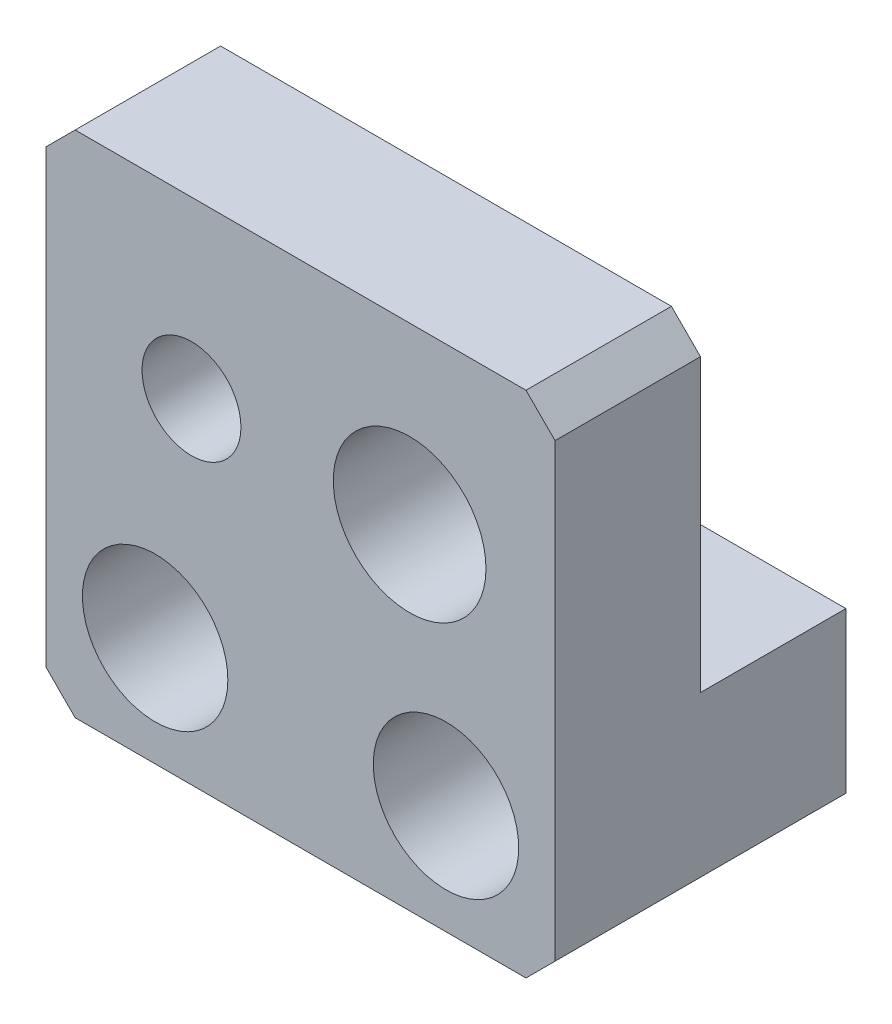
from build123d import *

# Parameters (mm, degrees)
SKETCH_1_W                   = 35
SKETCH_1_H                   = 35
EXTRUDE_1_DEPTH              = 20
CHAMFER_1_SIZE               = 2
M12X1_25_1_D                 = 10.5
HOLE_WIZARD_M8_1_D           = 6.8
HOLE_WIZARD_M5_1_D           = 5.5
HOLE_WIZARD_M5_1_CBORE_D     = 10
HOLE_WIZARD_M5_1_CBORE_DEPTH = 12
SKETCH_11_W                  = 10
SKETCH_11_H                  = 22
CUT_EXTRUDE_1_DEPTH          = 44.945989578


with BuildPart() as part:
    # 草图1 → 凸台-拉伸1 (new body)
    with BuildSketch(Plane.XY):
        Rectangle(SKETCH_1_W, SKETCH_1_H)
    extrude(amount=EXTRUDE_1_DEPTH)

    # 倒角1
    chamfer_1_edges = [part.edges().sort_by_distance(p)[0] for p in [
        (17.5, -17.5, 10),
        (-17.5, -17.5, 10),
        (-17.5, 17.5, 10),
        (17.5, 17.5, 10),
    ]]
    chamfer(chamfer_1_edges, length=CHAMFER_1_SIZE)

    # M12x1.25 螺纹孔1 (through all)
    with Locations(Plane.XY.offset(20)):
        with Locations((7.5, 5.5)):
            Hole(M12X1_25_1_D / 2)

    # M8 螺纹孔1 (through all)
    with Locations(Plane.XY.offset(20)):
        with Locations((-7.5, 5.5)):
            Hole(HOLE_WIZARD_M8_1_D / 2)

    # M5 六角圆柱头螺钉的柱形沉头孔1 (through all)
    with Locations(Plane.XY.offset(20)):
        with Locations((-10, -10), (10, -10)):
            CounterBoreHole(HOLE_WIZARD_M5_1_D / 2, HOLE_WIZARD_M5_1_CBORE_D / 2, HOLE_WIZARD_M5_1_CBORE_DEPTH)

    # 草图11 → 切除-拉伸1 (cut, through all)
    with BuildSketch(Plane(origin=(17.5, 0, 0), x_dir=(0, 0, -1), z_dir=(1, 0, 0))):
        with Locations((-5, 6.5)):
            Rectangle(SKETCH_11_W, SKETCH_11_H)
    extrude(amount=-CUT_EXTRUDE_1_DEPTH, mode=Mode.SUBTRACT)


solid = part.part
